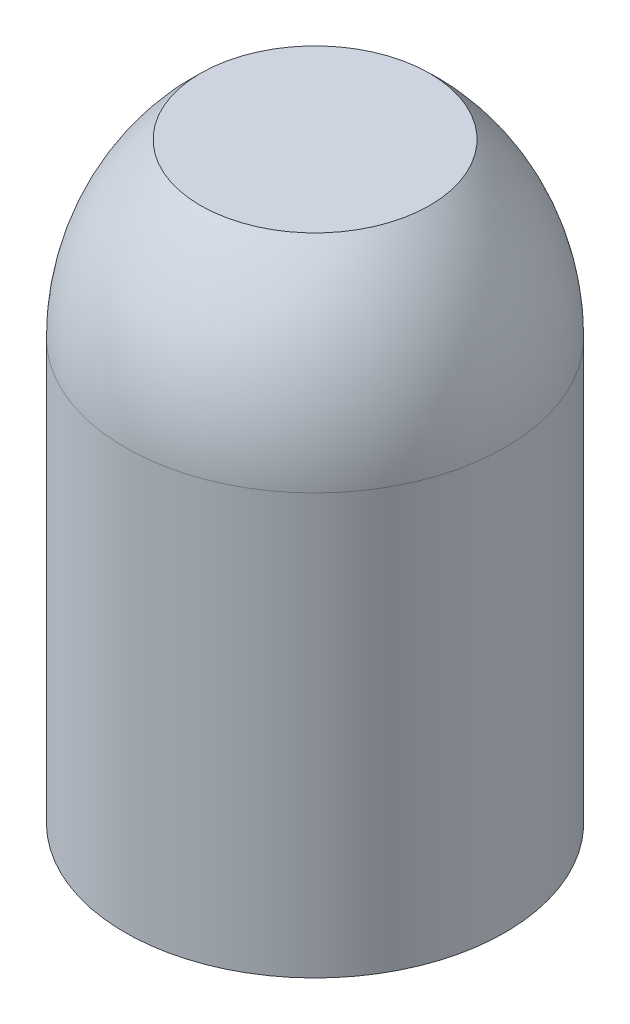
SolidWorks part; units mm, degrees
material "SUS304"
ref_plane "Front View" through (0, 0, 0) normal (0, 0, 1) x (1, 0, 0)
ref_plane "Top View" through (0, 0, 0) normal (0, 1, 0) x (1, 0, 0)
ref_plane "Right View" through (0, 0, 0) normal (1, 0, 0) x (0, 0, -1)
sketch "Sketch1" plane through (0, 0, 0) normal (0, 0, 1) x (1, 0, 0)
  line L0 (0, 0) -> (0, 34.6592) construction
  line L1 (0, 0) -> (-4.975, 0)
  line L2 (-4.975, 0) -> (-4.975, 11)
  line L3 (-3, 15.5) -> (0, 15.5)
  line L4 (0, 15.5) -> (0, 0)
  arc A0 (-4.975, 11) -> (-3, 15.5) centre (1.1391, 11) cw
  dimension "D1" = 9.95
  dimension "D2" = 11
  dimension "D3" = 4.5
  dimension "D4" = 6
revolve "Revolve1" add sketch "Sketch1" angle 360 about L0
hole_wizard "M3 Tapped Hole1" positions "Sketch2" profile "Sketch3" tap size "M3" standard "GB"
sketch "Sketch2" plane through (0, 0, 0) normal (0, -1, 0) x (-1, 0, 0)
  point P0 (0, 0)
sketch "Sketch3" plane through (0, 0, 0) normal (1, 0, 0) x (0, 0, -1)
  line L0 (0, 0) -> (0, 8.2511)
  line L1 (0, 8.2511) -> (1.25, 7.5)
  line L2 (1.25, 7.5) -> (1.25, 0)
  line L5 (1.25, 0) -> (0, 0)
  line L10 (0, 8.2511) -> (-1.25, 7.5) construction
  line L11 (0, -6.35) -> (0, 107.95) construction
  dimension "螺纹孔钻头直径" = 2.5
  dimension "螺纹孔钻头深度" = 7.5
  dimension "导头角度" = 118
cosmetic thread "Hole Thread1" parameters "D1"=6, "D2"=3
